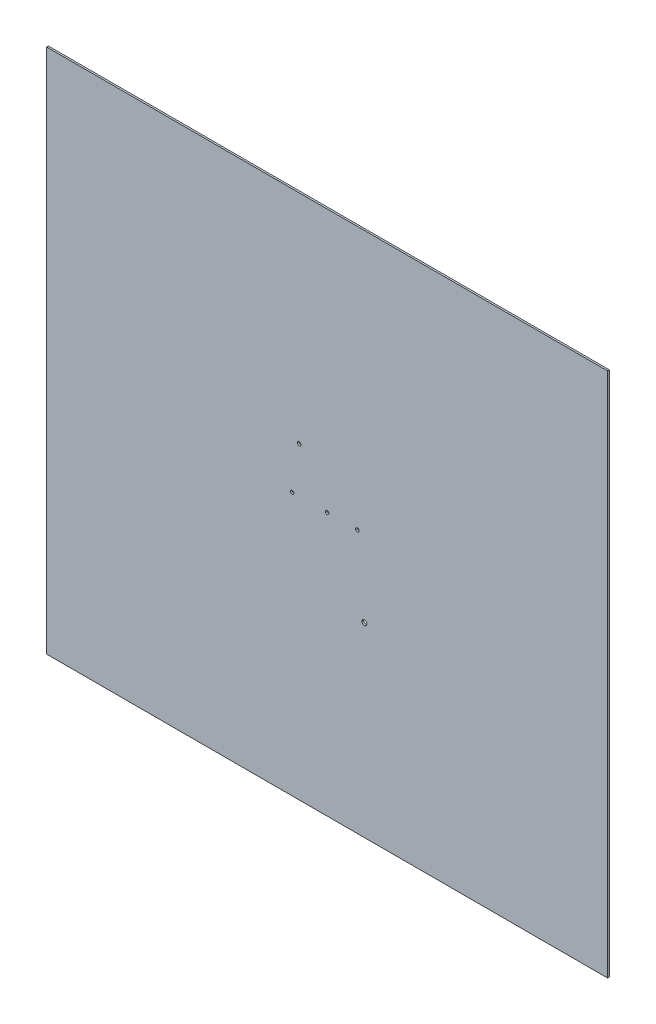
SolidWorks part; units mm, degrees
ref_plane "Front Plane" through (0, 0, 0) normal (0, 0, 1) x (1, 0, 0)
ref_plane "Top Plane" through (0, 0, 0) normal (0, 1, 0) x (1, 0, 0)
ref_plane "Right Plane" through (0, 0, 0) normal (1, 0, 0) x (0, 0, -1)
other "Configuration Table"
sketch "Sketch1" plane through (0, 0, 0) normal (0, 0, 1) x (1, 0, 0)
  line L0 (-800, 0) -> (800, 0) construction
  line L1 (-800, 750) -> (800, 750)
  line L2 (-800, 750) -> (-800, -750)
  line L3 (-800, -750) -> (800, -750)
  line L4 (800, 750) -> (800, -750)
  line L5 (-800, 750) -> (800, -750) construction
  line L6 (-800, -750) -> (800, 750) construction
  circle A0 centre (0, 0) radius 5
  circle A1 centre (-99.75, 0) radius 5
  circle A9 centre (86.25, 0) radius 5
  circle A10 centre (106.25, -219.089) radius 6.8655
  circle A11 centre (-79.75, 130) radius 5.0071
  point P0 (0, 0)
  dimension "D3" = 86.25
  dimension "D4" = 220
  dimension "D5" = 99.75
  dimension "D6" = 20
  dimension "D7" = 130
  dimension "D8" = 20
  dimension "D1" = 1600
  dimension "D2" = 1500
extrude "Boss-Extrude1" add sketch "Sketch1" along normal blind 5
